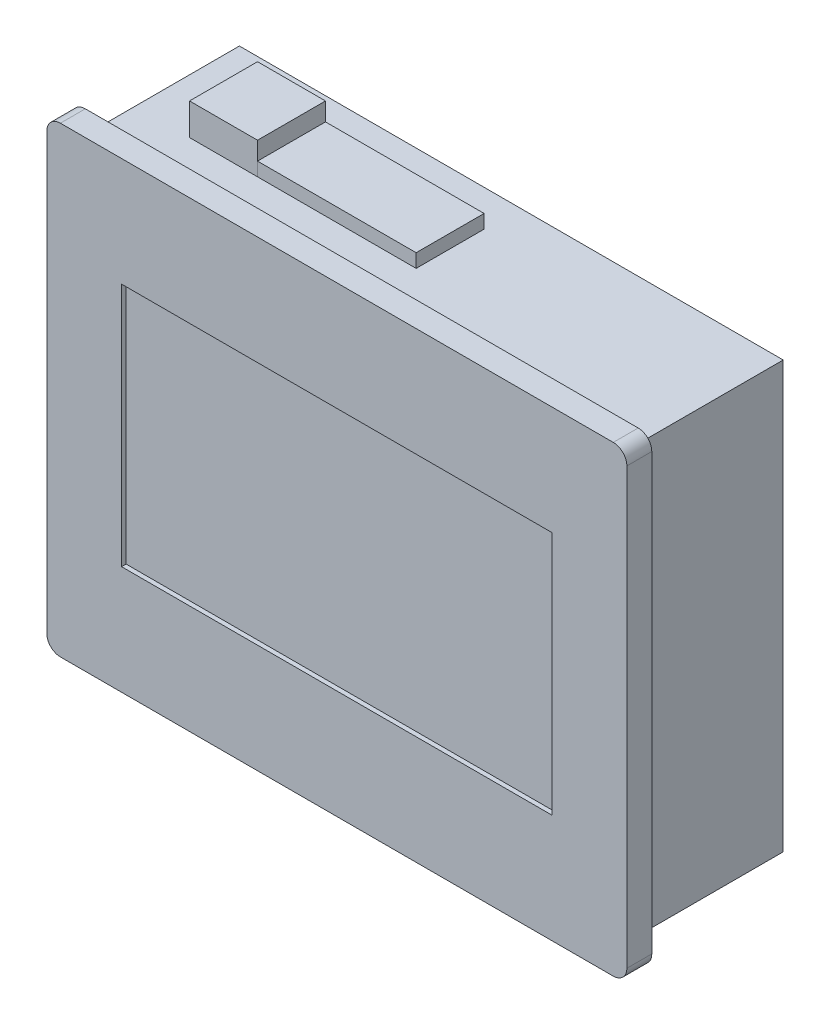
SolidWorks part; units mm, degrees
material "Polyurethane"
ref_plane "Front" through (0, 0, 0) normal (0, 0, 1) x (1, 0, 0)
ref_plane "Top" through (0, 0, 0) normal (0, 1, 0) x (1, 0, 0)
ref_plane "Right" through (0, 0, 0) normal (1, 0, 0) x (0, 0, -1)
sketch "Sketch1" plane through (0, 0, 0) normal (0, 0, 1) x (1, 0, 0)
  line L1 (64, -51) -> (-64, -51)
  line L2 (64, -51) -> (64, 51)
  line L3 (64, 51) -> (-64, 51)
  line L4 (-64, -51) -> (-64, 51)
  line L5 (64, -51) -> (-64, 51) construction
  line L6 (64, 51) -> (-64, -51) construction
  point P0 (0, 0)
  dimension "D1" = 102
  dimension "D2" = 128
extrude "Boss-Extrude1" add sketch "Sketch1" along normal blind 5.5
sketch "Sketch2" plane through (0, 0, 5.5) normal (0, 0, 1) x (1, 0, 0)
  line L1 (47.5, -27) -> (-47.5, -27)
  line L2 (47.5, -27) -> (47.5, 27)
  line L3 (47.5, 27) -> (-47.5, 27)
  line L4 (-47.5, -27) -> (-47.5, 27)
  line L5 (47.5, -27) -> (-47.5, 27) construction
  line L6 (47.5, 27) -> (-47.5, -27) construction
  point P0 (0, 0)
  dimension "D1" = 54
  dimension "D2" = 95
extrude "Cut-Extrude1" cut sketch "Sketch2" against normal blind 1
sketch "Sketch3" plane through (0, 0, 0) normal (0, 0, -1) x (-1, 0, 0)
  line L1 (60, -47) -> (-60, -47)
  line L2 (60, -47) -> (60, 47)
  line L3 (60, 47) -> (-60, 47)
  line L4 (-60, -47) -> (-60, 47)
  line L5 (60, -47) -> (-60, 47) construction
  line L6 (60, 47) -> (-60, -47) construction
  point P0 (0, 0)
  dimension "D1" = 94
  dimension "D2" = 120
extrude "Boss-Extrude2" add sketch "Sketch3" along normal blind 33
fillet "Fillet1" radius 3 4 edges at (-64, 51, 2.75) (64, 51, 2.75) (64, -51, 2.75) (-64, -51, 2.75)
sketch "Sketch4" plane through (0, 47, 0) normal (0, 1, 0) x (1, 0, 0)
  line L0 (-60, 0) -> (60, 0) construction
  line L1 (-48, 25) -> (-33, 25)
  line L2 (-48, 25) -> (-48, 10)
  line L3 (-48, 10) -> (-33, 10)
  line L4 (-33, 25) -> (-33, 10)
  line L5 (-60, 33) -> (-60, 0) construction
  point P4 (-40.5, 10)
  dimension "D1" = 15
  dimension "D2" = 15
  dimension "D3" = 10
  dimension "D4" = 12
extrude "Boss-Extrude3" add sketch "Sketch4" along normal blind 7
sketch "Sketch5" plane through (0, 47, 0) normal (0, 1, 0) x (1, 0, 0)
  line L1 (-33, 25) -> (2, 25)
  line L2 (-33, 25) -> (-33, 10)
  line L3 (-33, 10) -> (2, 10)
  line L4 (2, 25) -> (2, 10)
  dimension "D2" = 35
extrude "Boss-Extrude4" add sketch "Sketch5" along normal blind 3 separate body
